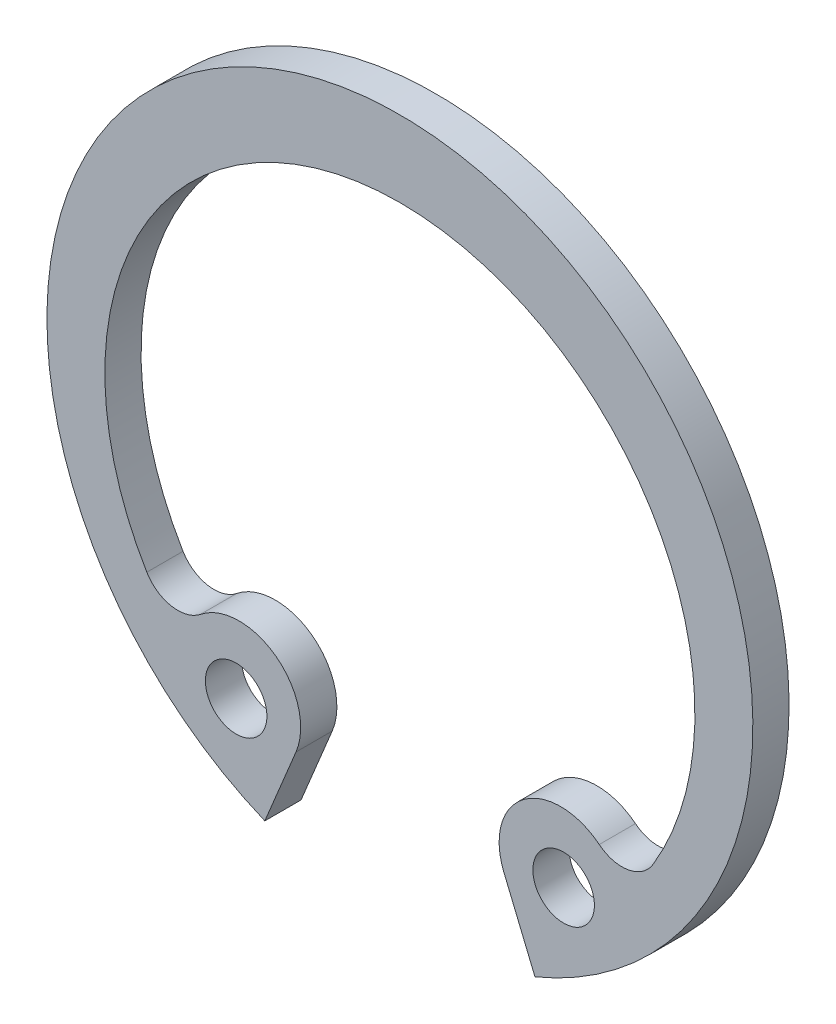
SolidWorks part; units mm, degrees
ref_plane "前视" through (0, 0, 0) normal (0, 0, 1) x (1, 0, 0)
ref_plane "上视" through (0, 0, 0) normal (0, 1, 0) x (1, 0, 0)
ref_plane "右视" through (0, 0, 0) normal (1, 0, 0) x (0, 0, -1)
sketch "尺寸草图" plane through (0, 0, 0) normal (0, 0, 1) x (1, 0, 0)
  line L0 (-9.75, 0) -> (9.75, 0) construction
  line L1 (0, 0) -> (-8.4437, -4.875) construction
  circle A0 centre (0, 0) radius 9.75
  point P5 (-6.55, 0)
  point P6 (6.9, 0)
  point P7 (1.7, 0)
  point P8 (7.9, 0)
  point P10 (-2.06, 0)
  point P11 (-0.5, 0)
  point P12 (-3.76, 0)
  point P13 (-7.55, 0)
  point P14 (30.5274, 17.625)
sketch "草图1" plane through (0, 0, 0) normal (0, 0, 1) x (1, 0, 0)
  line L0 (0, 9.75) -> (0, -9.0078) construction
  line L1 (-2.87, -6.9289) -> (-3.7312, -9.0078)
  line L2 (-4.6053, -6.6759) -> (-4.4406, -6.2783) construction
  line L3 (0, 0) -> (-3.7312, -9.0078) construction
  line L4 (2.87, -6.9289) -> (3.7312, -9.0078)
  arc A0 (3.7312, -9.0078) -> (-3.7312, -9.0078) centre (0, 0) ccw
  arc A1 (6.9912, -4.6888) -> (-6.9912, -4.6888) centre (0, -0.5) ccw
  circle A2 centre (-4.523, -6.4771) radius 0.85
  arc A3 (-2.87, -6.9289) -> (-5.5064, -4.9539) centre (-4.4406, -6.2783) ccw
  arc A4 (-5.5064, -4.9539) -> (-6.9912, -4.6888) centre (-6.1334, -4.1748) cw
  circle A5 centre (4.523, -6.4771) radius 0.85
  arc A6 (2.87, -6.9289) -> (5.5064, -4.9539) centre (4.4406, -6.2783) cw
  arc A7 (5.5064, -4.9539) -> (6.9912, -4.6888) centre (6.1334, -4.1748) ccw
extrude "基体-拉伸" add sketch "草图1" along normal blind 1
equation "\"D1@草图1\" = \"DD@尺寸草图\" "
equation "\"D2@草图1\"=\"d@尺寸草图\""
equation "\"D3@草图1\" = \"c@尺寸草图\""
equation "\"D6@草图1\" = \"RR@尺寸草图\""
equation "\"D8@草图1\" = \"R2@尺寸草图\""
equation "\"D7@草图1\" = \"R1@尺寸草图\""
equation "\"D4@草图1\" = \"aa@尺寸草图\"/2"
equation "\"D9@草图1\" = \"a@尺寸草图\""
equation "\"D5@草图1\" = \"d1@尺寸草图\""
equation "\"D1@基体-拉伸\" = \"s@尺寸草图\"/2"
equation "\"D2@基体-拉伸\" = \"D1@基体-拉伸\""
